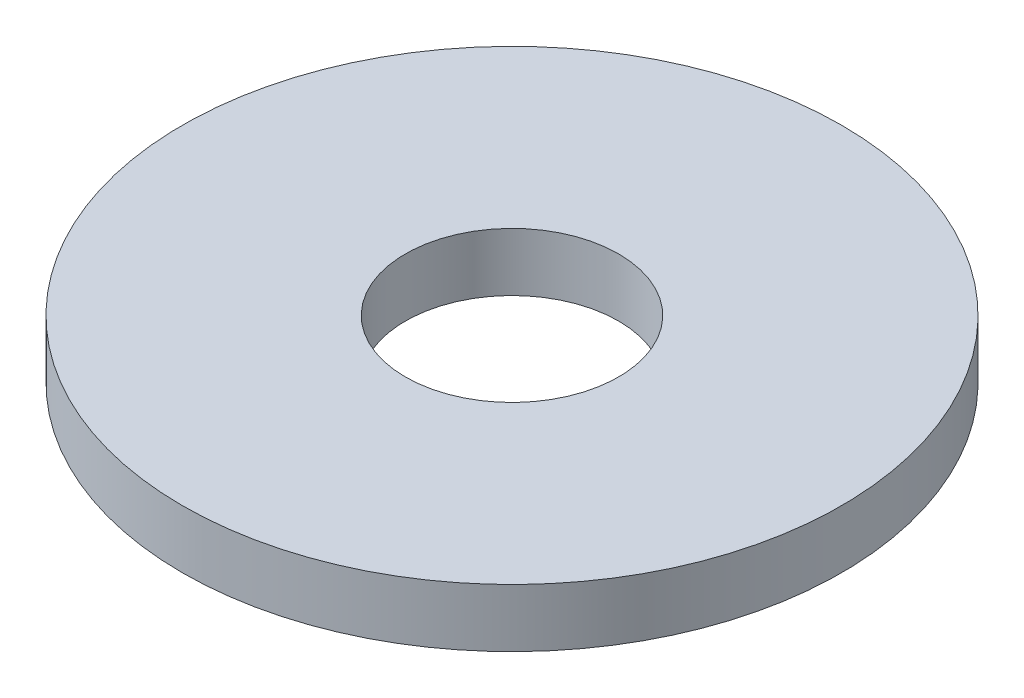
SolidWorks part; units mm, degrees
material "钢"
ref_plane "基准面1" through (0, 0, 0) normal (0, 0, 1) x (1, 0, 0)
ref_plane "基准面2" through (0, 0, 0) normal (0, 1, 0) x (1, 0, 0)
ref_plane "基准面3" through (0, 0, 0) normal (1, 0, 0) x (0, 0, -1)
sketch "尺寸草图" plane through (0, 0, 0) normal (0, 0, 1) x (1, 0, 0)
  line L0 (0, 0) -> (9.1, 0)
  point P3 (3, 0)
  point P4 (34, 0)
  point P5 (11, 0)
sketch "草图1" plane through (0, 0, 0) normal (0, 0, 1) x (1, 0, 0)
  line L0 (0, 0) -> (0, 52.7318) construction
  line L2 (-5.5, 8.6445) -> (-17, 8.6445)
  line L3 (-5.5, 8.6445) -> (-5.5, 11.6445)
  line L4 (-5.5, 11.6445) -> (-17, 11.6445)
  line L5 (-17, 8.6445) -> (-17, 11.6445)
revolve "基体-旋转" add sketch "草图1" angle 360 about L0
equation "\"h@草图1\" = \"h@尺寸草图\""
equation "\"D1@草图1\" = \"d1@尺寸草图\" / 2"
equation "\"D2@草图1\" = \"d2@尺寸草图\" / 2"
